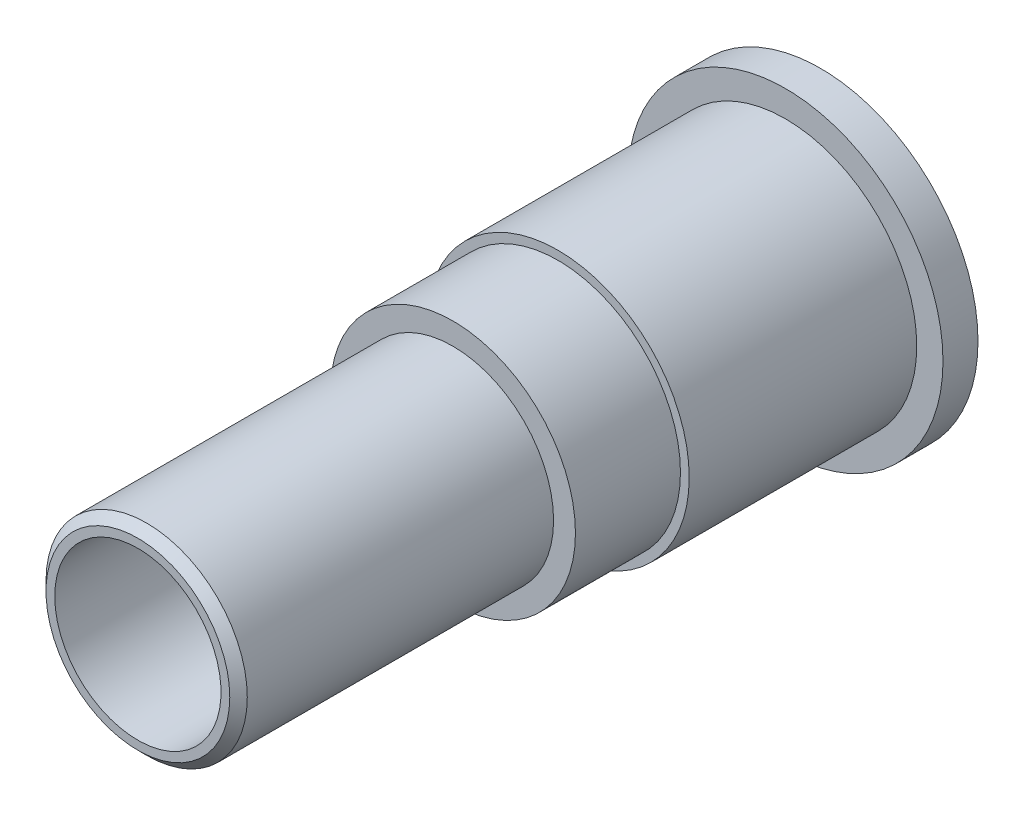
SolidWorks part; units mm, degrees
ref_plane "Front Plane" through (0, 0, 0) normal (0, 0, 1) x (1, 0, 0)
ref_plane "Top Plane" through (0, 0, 0) normal (0, 1, 0) x (1, 0, 0)
ref_plane "Right Plane" through (0, 0, 0) normal (1, 0, 0) x (0, 0, -1)
sketch "Sketch1" plane through (0, 0, 0) normal (0, 0, 1) x (1, 0, 0)
  circle A0 centre (0, 0) radius 9
  dimension "D1" = 18
extrude "Boss-Extrude1" add sketch "Sketch1" along normal blind 2
sketch "Sketch2" plane through (0, 0, 2) normal (0, 0, 1) x (1, 0, 0)
  circle A0 centre (0, 0) radius 7.5
  dimension "D1" = 15
extrude "Boss-Extrude2" add sketch "Sketch2" along normal blind 13
sketch "Sketch3" plane through (0, 0, 15) normal (0, 0, 1) x (1, 0, 0)
  circle A0 centre (0, 0) radius 7
  dimension "D1" = 14
extrude "Boss-Extrude3" add sketch "Sketch3" along normal blind 6
cosmetic thread "Cosmetic Thread1" parameters "D2"=12.376
sketch "Sketch5" plane through (0, 0, 21) normal (0, 0, 1) x (1, 0, 0)
  circle A0 centre (0, 0) radius 5.75
  dimension "D1" = 11.5
extrude "Boss-Extrude4" add sketch "Sketch5" along normal blind 18
sketch "Sketch4" plane through (0, 0, 0) normal (0, 0, -1) x (-1, 0, 0)
  circle A0 centre (0, 0) radius 4.75
  dimension "D1" = 9.5
extrude "Cut-Extrude1" cut sketch "Sketch4" against normal through all
chamfer "Chamfer1" distance 0.5 angle 45 1 edges at (5.75, 0, 39)
chamfer "Chamfer2" distance 0.3 distance2 10 1 edges at (-4.75, 0, 0)
